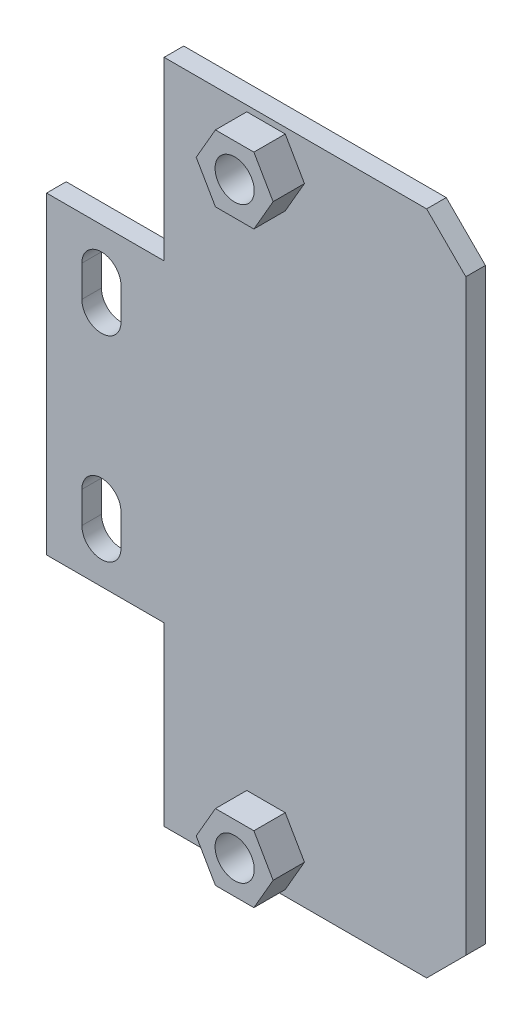
SolidWorks part; units mm, degrees
material "Q235-A"
ref_plane "前视基准面" through (0, 0, 0) normal (0, 0, 1) x (1, 0, 0)
ref_plane "上视基准面" through (0, 0, 0) normal (0, 1, 0) x (1, 0, 0)
ref_plane "右视基准面" through (0, 0, 0) normal (1, 0, 0) x (0, 0, -1)
sketch "草图1" plane through (0, 0, 0) normal (0, 0, 1) x (1, 0, 0)
  line L1 (-26, 85) -> (26, 85)
  line L2 (-26, 85) -> (-26, -85)
  line L3 (-26, -85) -> (26, -85)
  line L4 (26, 85) -> (26, -85)
  line L5 (-26, 85) -> (26, -85) construction
  line L6 (-26, -85) -> (26, 85) construction
  circle A0 centre (0, 75) radius 6.25
  circle A1 centre (0, -75) radius 6.25
  point P0 (0, 0)
  dimension "D3" = 75
  dimension "D4" = 75
  dimension "D6" = 12.5
  dimension "D1" = 170
  dimension "D2" = 52
extrude "凸台-减震垫孔" add sketch "草图1" along normal blind 5
sketch "草图6" plane through (0, 0, 0) normal (0, 0, -1) x (-1, 0, 0)
  line L0 (26, 85) -> (26, -85) construction
  line L1 (26, 40) -> (56, 40)
  line L2 (26, 40) -> (26, -40)
  line L3 (26, -40) -> (56, -40)
  line L4 (56, 40) -> (56, -40)
  line L5 (-26, 85) -> (26, 85) construction
  line L6 (26, -85) -> (-26, -85) construction
  dimension "D1" = 45
  dimension "D2" = 45
  dimension "D3" = 30
extrude "凸台-梁孔" add sketch "草图6" against normal up to surface (5 mm away) up to face at (6.25, 75, 5)
sketch "草图10" plane through (0, 0, 5) normal (0, 0, 1) x (1, 0, 0)
  line L0 (-42, -29) -> (-42, -21) construction
  line L1 (-47, -29) -> (-47, -21)
  line L2 (-37, -29) -> (-37, -21)
  line L3 (-63.0022, 0) -> (10.7371, 0) construction
  line L4 (-42, 29) -> (-42, 21) construction
  line L5 (-47, 29) -> (-47, 21)
  line L6 (-37, 29) -> (-37, 21)
  arc A0 (-47, -29) -> (-37, -29) centre (-42, -29) ccw
  arc A1 (-37, -21) -> (-47, -21) centre (-42, -21) ccw
  arc A2 (-47, 29) -> (-37, 29) centre (-42, 29) cw
  arc A3 (-37, 21) -> (-47, 21) centre (-42, 21) cw
  point P2 (-42, -25)
  point P12 (-42, 25)
  dimension "D2" = 5
  dimension "D1" = 8
  dimension "D3" = 50
  dimension "D4" = 42
extrude "切除-梁孔" cut sketch "草图10" against normal through all
sketch "草图3" plane through (0, 0, 5) normal (0, 0, 1) x (1, 0, 0)
  line L1 (9.815, 75) -> (4.9075, 83.5)
  line L2 (4.9075, 83.5) -> (-4.9075, 83.5)
  line L3 (-4.9075, 83.5) -> (-9.815, 75)
  line L4 (-9.815, 75) -> (-4.9075, 66.5)
  line L5 (-4.9075, 66.5) -> (4.9075, 66.5)
  line L6 (4.9075, 66.5) -> (9.815, 75)
  line L7 (9.815, -75) -> (4.9075, -66.5)
  line L8 (4.9075, -66.5) -> (-4.9075, -66.5)
  line L9 (-4.9075, -66.5) -> (-9.815, -75)
  line L10 (-9.815, -75) -> (-4.9075, -83.5)
  line L11 (-4.9075, -83.5) -> (4.9075, -83.5)
  line L12 (4.9075, -83.5) -> (9.815, -75)
  circle A0 centre (0, 75) radius 8.5 construction
  circle A1 centre (0, 75) radius 5
  circle A2 centre (0, -75) radius 8.5 construction
  circle A3 centre (0, -75) radius 5
  dimension "D1" = 17
  dimension "D2" = 10
  dimension "D3" = 17
  dimension "D4" = 10
extrude "凸台-拉伸2" add sketch "草图3" along normal blind 8 separate body
sketch "草图11" plane through (0, 0, 5) normal (0, 0, 1) x (1, 0, 0)
  line L1 (26, -85) -> (51, -85)
  line L2 (26, -85) -> (26, 85)
  line L3 (26, 85) -> (51, 85)
  line L4 (51, -85) -> (51, 85)
  dimension "D1" = 25
extrude "凸台-拉伸3" add sketch "草图11" against normal up to surface (5 mm away) separate body up to face at (-42, -25, 0)
combine bodies "组合1" operation type add bodies to combine 111 112
chamfer "倒角6" distance 10 angle 45 2 edges at (51, 85, 2.5) (51, -85, 2.5)
equation "\"BH\"= \"D1@凸台-减震垫孔\""
